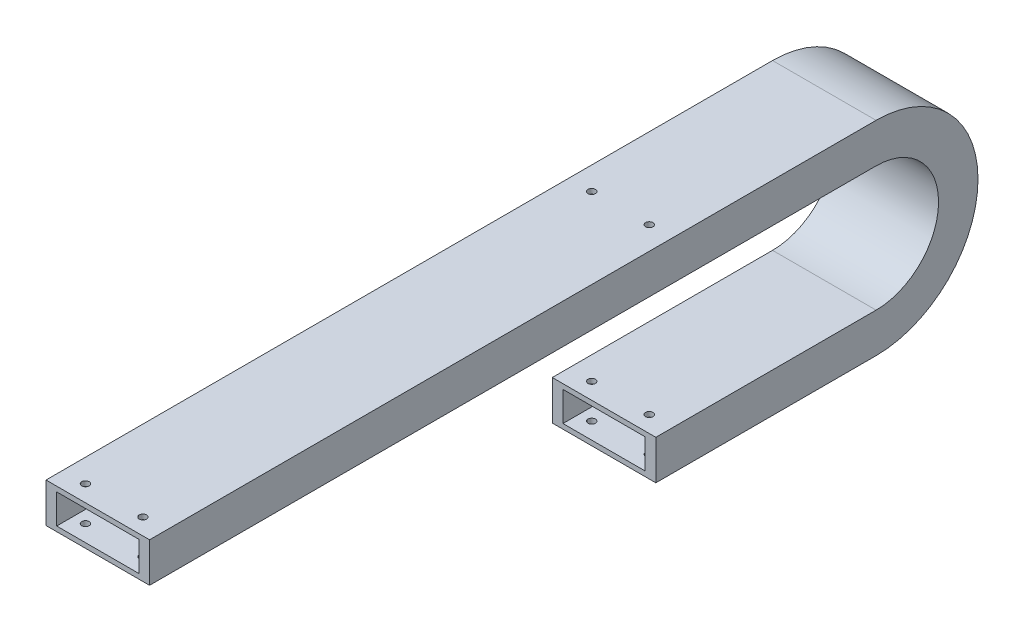
SolidWorks part; units mm, degrees
ref_plane "前视基准面" through (0, 0, 0) normal (0, 0, 1) x (1, 0, 0)
ref_plane "上视基准面" through (0, 0, 0) normal (0, 1, 0) x (1, 0, 0)
ref_plane "右视基准面" through (0, 0, 0) normal (1, 0, 0) x (0, 0, -1)
sketch "草图1" plane through (0, 0, 0) normal (0, 0, 1) x (1, 0, 0)
  line L1 (25, -9) -> (-25, -9)
  line L2 (25, -9) -> (25, 9)
  line L3 (25, 9) -> (-25, 9)
  line L4 (-25, -9) -> (-25, 9)
  line L5 (25, -9) -> (-25, 9) construction
  line L6 (25, 9) -> (-25, -9) construction
  line L7 (31.5, -12) -> (-31.5, -12)
  line L8 (31.5, -12) -> (31.5, 12)
  line L9 (31.5, 12) -> (-31.5, 12)
  line L10 (-31.5, -12) -> (-31.5, 12)
  line L11 (31.5, -12) -> (-31.5, 12) construction
  line L12 (31.5, 12) -> (-31.5, -12) construction
  point P0 (0, 0)
  point P6 (0, 0)
  dimension "D1" = 18
  dimension "D2" = 24
  dimension "D3" = 50
  dimension "D4" = 63
sketch "草图2" plane through (0, 0, 0) normal (1, 0, 0) x (0, 0, -1)
  line L0 (0, 0) -> (134, 0)
  line L1 (134, 100) -> (-308, 100)
  arc A0 (134, 0) -> (134, 100) centre (134, 50) ccw
  dimension "D3" = 50
  dimension "D1" = 134
  dimension "D2" = 442
sweep "扫描1" add profiles "草图1" path "草图2"
sketch "草图5" plane through (0, -12, 0) normal (0, -1, 0) x (1, 0, 0)
  line L0 (31.5, 308) -> (-31.5, 308) construction
  line L1 (-31.5, -134) -> (-31.5, 308) construction
  line L2 (-31.5, 0) -> (31.5, 0) construction
  circle A0 centre (-17.5, -10) radius 2.25
  circle A1 centre (17.5, -10) radius 2.25
  circle A2 centre (-17.5, 298) radius 2.25
  circle A3 centre (17.5, 298) radius 2.25
  dimension "D1" = 35
  dimension "D2" = 4.5
  dimension "D3" = 10
  dimension "D4" = 14
  dimension "D5" = 10
extrude "切除-拉伸3" cut sketch "草图5" against normal through all
